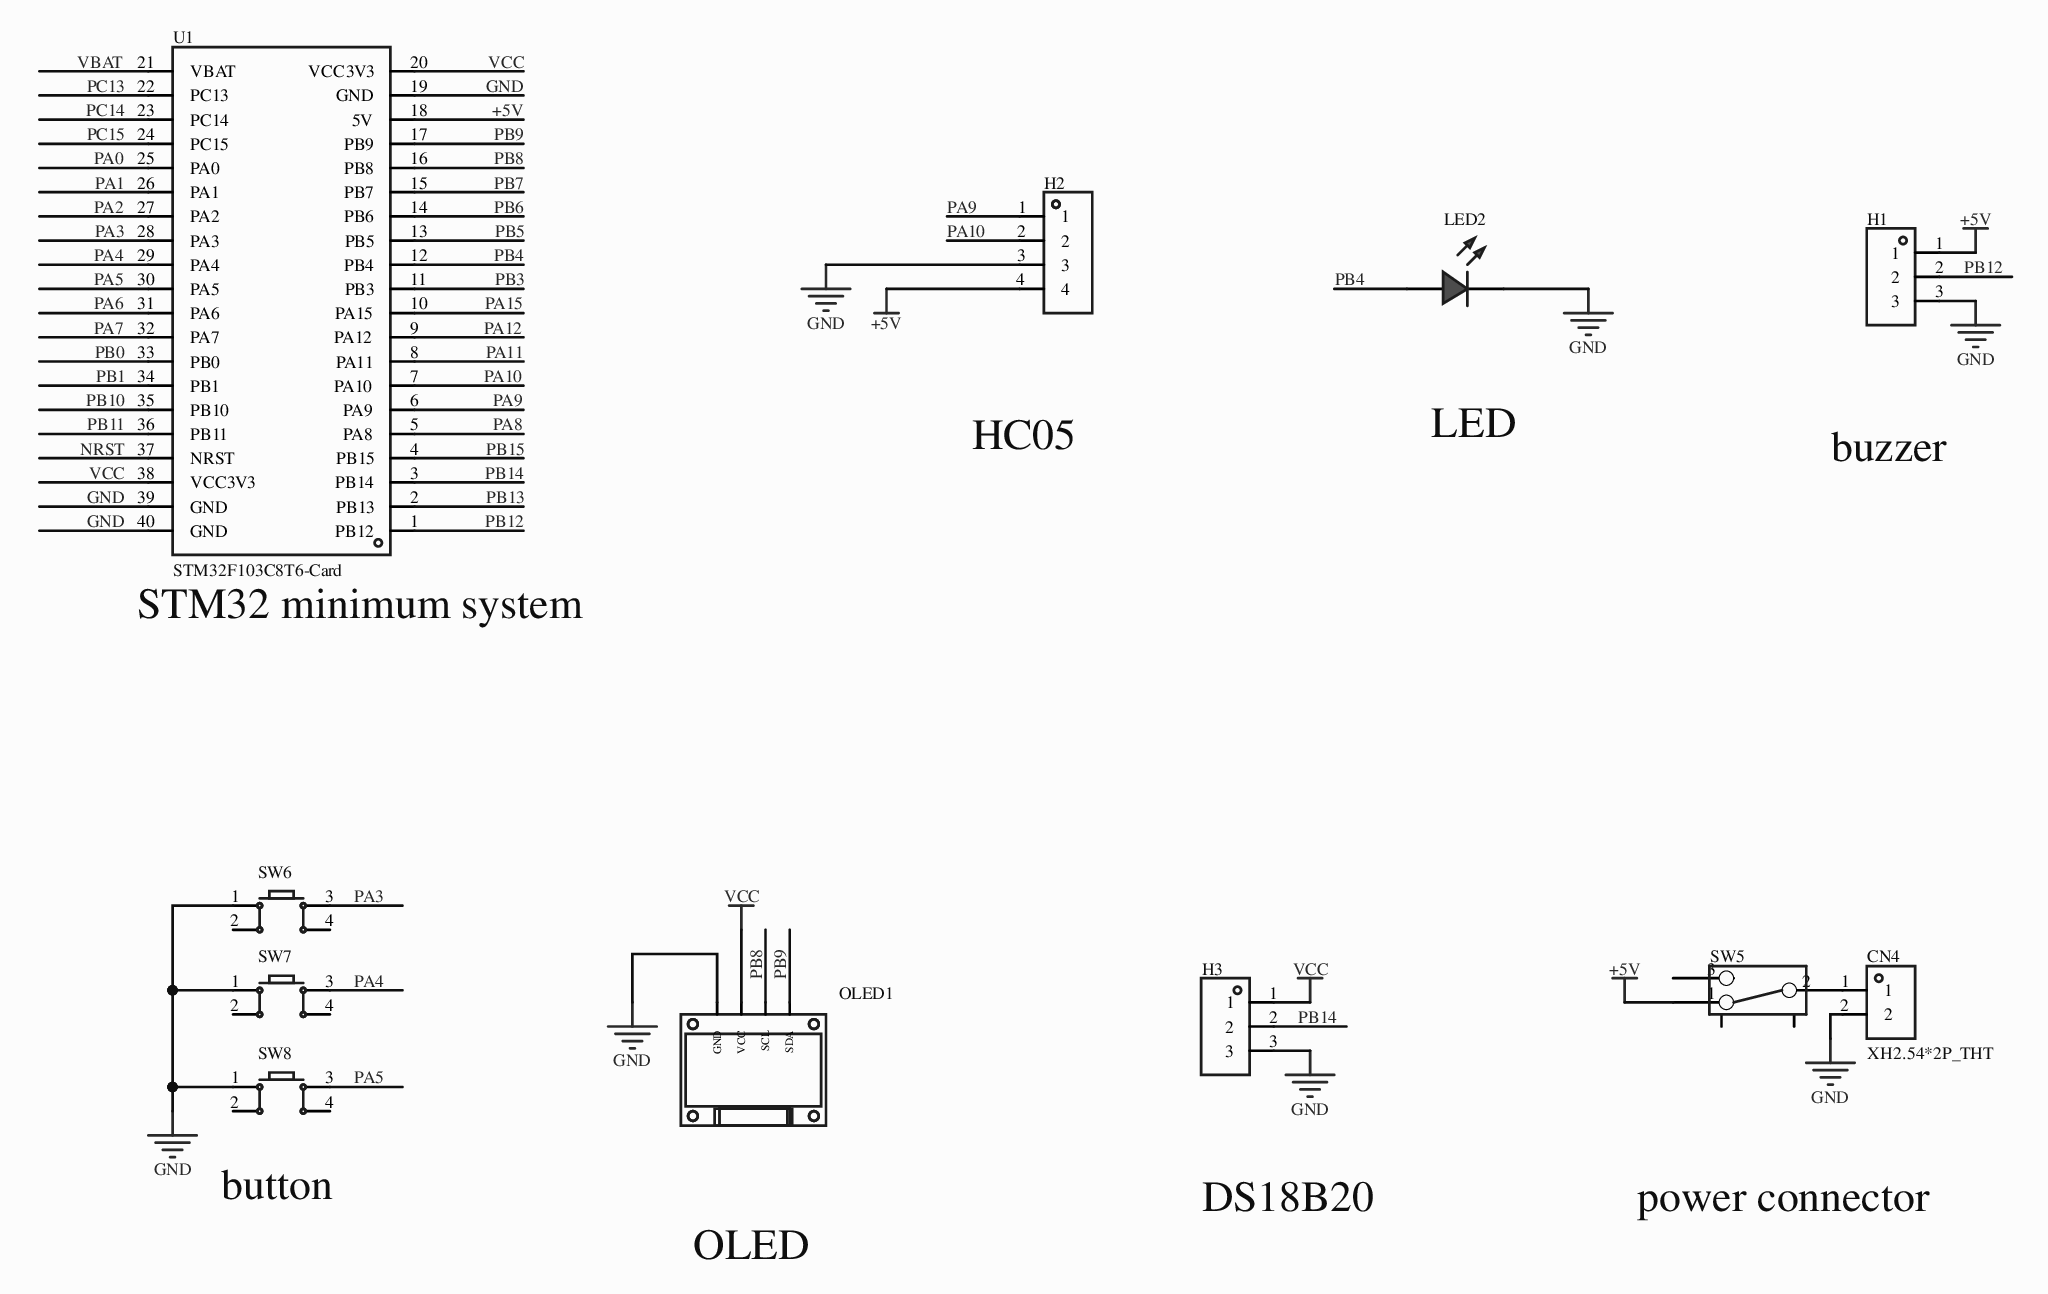
[diagram p0: MISC89015-3.schdoc]
# Altium project MISC89015-2.PrjPcb
1 sheet, 11 parts. Net scope: global (net labels, ports and power ports of the same name join across sheets).
Board file: MISC89015.pcbdoc

## Sheet MISC89015-3.schdoc
size 297 x 209 mm; Version: V1.0; @Project Name: MISC89015; @Page Count: 1; @Update Date: 2026-04-23; @Create Date: 2026-04-23; @Schematic Name: MISC89015; @Page No: 1; @Create Time: 23:22:16; @Update Time: 17:32:40; @Board Name: MISC89015

### Parts
CN4  XH2.54*2P_THT  [CONN-TH_2P-P2.50-XH2.54-2P]
H1  (no value)  [HDR-TH_3P-P2.54-V-F]
H2  (no value)  [HDR-TH_4P-P2.54-V-F]
H3  (no value)  [HDR-TH_3P-P2.54-V-F]
LED2  (no value)  [LED-TH_5mm]
OLED1  (no value)  [0.96OLED_4P]
SW5  (no value)  [拨动开关]
SW6  (no value)  [SW-TH_4P-L6.0-W6.0-P4.50-LS6.5]
SW7  (no value)  [SW-TH_4P-L6.0-W6.0-P4.50-LS6.5]
SW8  (no value)  [SW-TH_4P-L6.0-W6.0-P4.50-LS6.5]
U1  STM32F103C8T6-Card  [CONN-TH_L53.3-W22.9_STM32F103C8T6-CARD]

### Nets
+5V: H1.1 H2.4 SW5.1 U1.18(5V)
GND: CN4.2 H1.3 H2.3 H3.3 LED2.2(A) OLED1.1(GND) SW6.1 SW7.1 SW8.1 U1.19(GND) U1.39(GND) U1.40(GND)
VCC: H3.1 OLED1.2(VCC) U1.20(VCC3V3) U1.38(VCC3V3)
NRST: U1.37(NRST)
PA0: U1.25(PA0)
PA1: U1.26(PA1)
PA2: U1.27(PA2)
PA3: SW6.3 U1.28(PA3)
PA4: SW7.3 U1.29(PA4)
PA5: SW8.3 U1.30(PA5)
PA6: U1.31(PA6)
PA7: U1.32(PA7)
PA8: U1.5(PA8)
PA9: H2.1 U1.6(PA9)
PA10: H2.2 U1.7(PA10)
PA11: U1.8(PA11)
PA12: U1.9(PA12)
PA15: U1.10(PA15)
PB0: U1.33(PB0)
PB1: U1.34(PB1)
PB3: U1.11(PB3)
PB4: LED2.1(C) U1.12(PB4)
PB5: U1.13(PB5)
PB6: U1.14(PB6)
PB7: U1.15(PB7)
PB8: OLED1.3(SCL) U1.16(PB8)
PB9: OLED1.4(SDA) U1.17(PB9)
PB10: U1.35(PB10)
PB11: U1.36(PB11)
PB12: H1.2 U1.1(PB12)
PB13: U1.2(PB13)
PB14: H3.2 U1.3(PB14)
PB15: U1.4(PB15)
PC13: U1.22(PC13)
PC14: U1.23(PC14)
PC15: U1.24(PC15)
VBAT: U1.21(VBAT)
NetCN4_1: CN4.1 SW5.2

Not connected (* = marked no-connect by the designer): SW5 3 4 5; SW6 2 4; SW7 2 4; SW8 2 4

### Notes on the sheet
- HC05
- LED
- buzzer
- (near U1) STM32 minimum system
- (near SW8) button
- DS18B20
- power connector
- OLED

### Library data of the parts
CN4 = XH2.54*2P_直插: 3D Model: 325c595e30db4df8abe76612dd40b0fa0819f05c4eef4c71ace90d822a990e87; 3D Model Transform: 295.275,228.346,0,180,0,0,-0.002,-20.079,-137.795; AddInBom: yes; Device: XH2.54*2P_THT; Symbol: XH2.54*2P_THT; LCSC Part Name: XH2.54*2P_直插; Supplier Part: C9900008615; Manufacturer Part: XH2.54*2P_直插; Supplier Footprint: XH2.54_2P; JLCPCB Part Class: Extended Part; Supplier: LCSC; FootprintName: CONN-TH_2P-P2.50-XH2.54-2P; ConvertToPcb: yes; ModelName: CONN-TH_2P-P2.50-XH2.54-2P
H1 H3 = HDR-F_2.54_1x3P: Symbol: PM254V-11-03-H85; 3D Model: f3b3cc5aae9641bf9e56fc160cef875b; 3D Model Transform: 299.9994,100,0,0,0,0,0,0,-118.11; ConvertToPcb: yes; ModelName: HDR2.54-F-LI-1X3P; Device: HDR-F_2.54_1x3P; Supplier Part: C541850; Supplier Footprint: 插件; FootprintName: HDR-TH_3P-P2.54-V-F; AddInBom: yes
H2 = HDR-F_2.54_1x4P: Symbol: 2.54-1*4P female; ConvertToPcb: yes; ModelId: d187812051054f85879fcaa51a310d8e0819f05c4eef4c71ace90d822a990e87; ModelTransform: 419.6842,98.464,0,0,0,0,0,0,-118.11; Device: HDR-F_2.54_1x4P; FootprintName: HDR-TH_4P-P2.54-V-F; AddInBom: yes; SupplierPart: C2718488; Supplier Footprint: 插件; ModelName: HDR-TH_4P-P2.54-V-F
LED2 = LED_TH-R_5mm: 3D Model: fe9cea1bdf7642cd8d9a5077ed0e2b580819f05c4eef4c71ace90d822a990e87; 3D Model Transform: 222.16,238.98,581.81,180,0,0,-6,0,-220; ConvertToPcb: yes; ModelName: LED-TH_BD5.9-P2.54-RD_RED; Symbol: LED_TH-R; Device: LED_TH-R_5mm; Supplier Footprint: 插件; AddInBom: yes; FootprintName: LED-TH_5mm
OLED1 = 0.96OLED模块_4P: Device: 0.96OLED module_4P; ConvertToPcb: yes; ModelId: 79c000fdb68d45a296c2e9bedf4f9055; ModelTransform: 1393.69792,1318.895,0,0,0,0,0,-560.079,-137.795; Symbol: 0.96OLED module_4P; FootprintName: 0.96OLED_4P; AddInBom: yes; Supplier Footprint: 插件; ModelName: 0.96OLED_4P
SW5 = 拨动开关_正: Device: toggle switch_pos; Symbol: toggle switch; ConvertToPcb: yes; ModelId: 4321fe59a4074cbfb4989553f297c68f0819f05c4eef4c71ace90d822a990e87; ModelName: SW-TH_SS-12D02-VG4; ModelTransform: 370.09,208.7,472.35,0,0,0,0,0,-110; FootprintName: toggle switch; AddInBom: yes; Supplier Footprint: 插件
SW6-SW8 = Key_TH_6x6x6: Contact current: 50mA; rated voltage (DC): 12V; insulation resistance: 100MΩ; circuit structure: SPST; mounting: through-hole; button shape: round button; button/cap colour: black; actuation force: 260gf@±30gf; operating temperature: -25℃~+70℃; pin style: PC pin; switch length: 6mm; switch width: 6mm; switch height: 6mm; with bracket: no;; Symbol: tactile button; 3D Model: 20eee248bc684ccd8cbdbb1d0d91ec6f0819f05c4eef4c71ace90d822a990e87; 3D Model Transform: 236.22,323.03,0,90,0,0,0,0,-137.795; AddInBom: yes; ModelName: SW-TH_4P-L6.0-W6.0-H5.0-LS6.5-P4.50; Device: Key_TH_6x6x6; Supplier Footprint: 插件; FootprintName: SW-TH_4P-L6.0-W6.0-P4.50-LS6.5; ConvertToPcb: yes
U1 = STM32F103C8T6-Card: AddInBom: yes; Device: STM32F103C8T6-Card; Symbol: STM32F103C8T6-CARD; FootprintName: CONN-TH_L53.3-W22.9_STM32F103C8T6-CARD; LCSC Part Name: STM32F103C8T6-Card; SupplierPart: C9900077949; ManufacturerPart: STM32F103C8T6-Card; Supplier Footprint: 插件; Supplier: LCSC; ConvertToPcb: yes